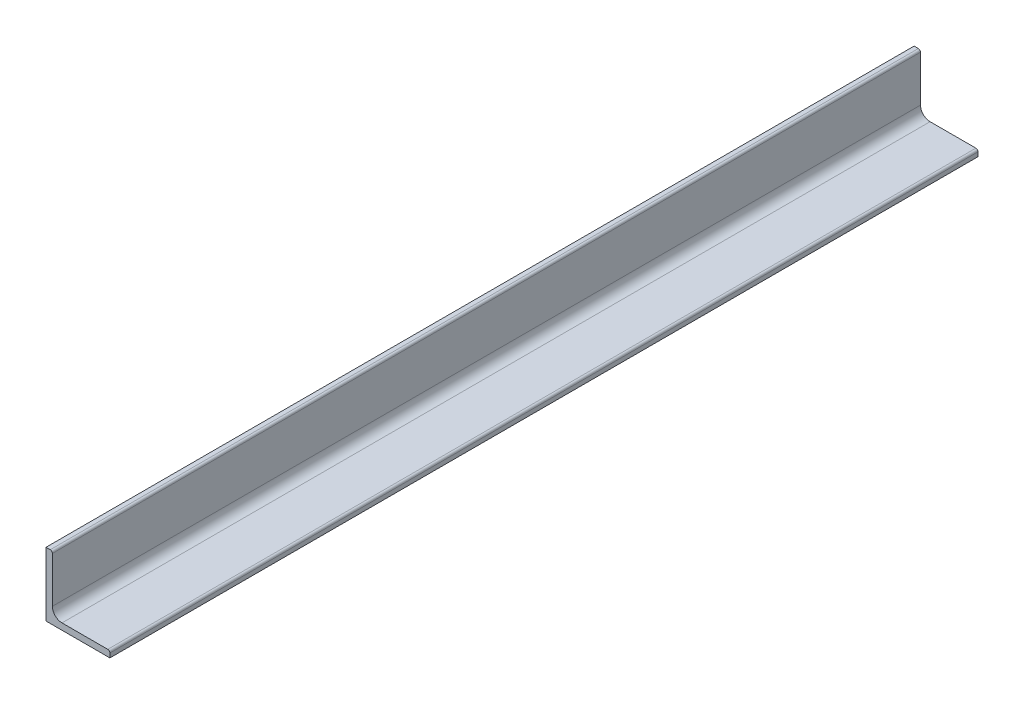
SolidWorks part; units mm, degrees
material "Plain Carbon Steel"
ref_plane "Plane1" through (0, 0, 0) normal (0, 0, 1) x (1, 0, 0)
ref_plane "Plane2" through (0, 0, 0) normal (0, 1, 0) x (1, 0, 0)
ref_plane "Plane3" through (0, 0, 0) normal (1, 0, 0) x (0, 0, -1)
sketch "Sketch1" plane through (0, 0, 0) normal (0, 0, 1) x (1, 0, 0)
  line L0 (0, 0) -> (0, 30)
  line L1 (0, 15) -> (3, 15) construction
  line L2 (3, 29) -> (3, 7.5)
  line L3 (7.5, 3) -> (29, 3)
  line L4 (15, 3) -> (15, 0) construction
  line L5 (30, 0) -> (0, 0)
  line L6 (0, 30) -> (2, 30)
  line L7 (30, 0) -> (30, 2)
  arc A0 (30, 2) -> (29, 3) centre (29, 2) ccw
  arc A1 (2, 30) -> (3, 29) centre (2, 29) cw
  arc A2 (7.5, 3) -> (3, 7.5) centre (7.5, 7.5) cw
  point P10 (15, 0)
  point P14 (0, 15)
  point P15 (3, 15)
  point P16 (15, 3)
  point P17 (3, 30)
  point P18 (30, 3)
  point P21 (30, 3)
  point P24 (3, 30)
extrude "Boss-Extrude1" add sketch "Sketch1" along normal mid plane 407.6 contours L2 A2 L3 A0 L7 L5 L0 L6 A1
equation "\"D2@Sketch1\" = \"D1@Sketch1\" / 3"
